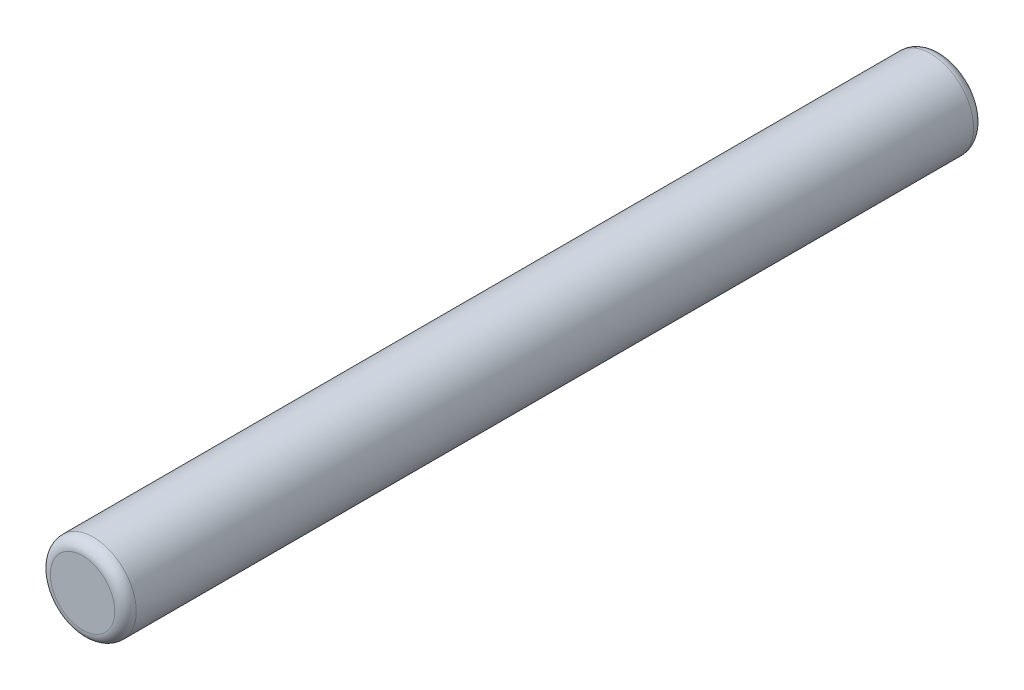
SolidWorks part; units mm, degrees
ref_plane "Front Plane" through (0, 0, 0) normal (0, 0, 1) x (1, 0, 0)
ref_plane "Top Plane" through (0, 0, 0) normal (0, 1, 0) x (1, 0, 0)
ref_plane "Right Plane" through (0, 0, 0) normal (1, 0, 0) x (0, 0, -1)
sketch "Sketch1" plane through (0, 0, 0) normal (0, 0, 1) x (1, 0, 0)
  circle A0 centre (-290, 235) radius 20 construction
  circle A1 centre (-290, 235) radius 20
extrude "Boss-Extrude1" add sketch "Sketch1" along normal blind 20 and the other way blind 380
fillet "Fillet1" radius 5 2 edges at (-270, 235, -380) (-270, 235, 20)
